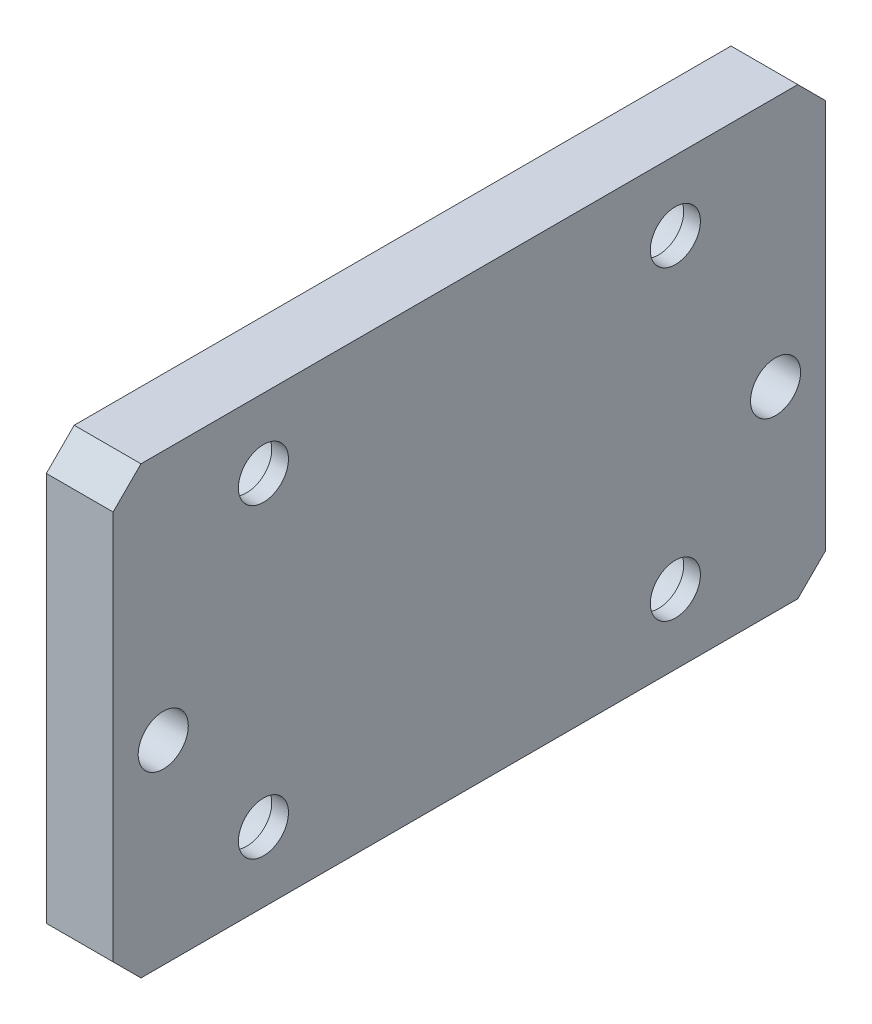
SolidWorks part; units mm, degrees
ref_plane "前视基准面" through (0, 0, 0) normal (0, 0, 1) x (1, 0, 0)
ref_plane "上视基准面" through (0, 0, 0) normal (0, 1, 0) x (1, 0, 0)
ref_plane "右视基准面" through (0, 0, 0) normal (1, 0, 0) x (0, 0, -1)
sketch "草图1" plane through (0, 0, 0) normal (1, 0, 0) x (0, 0, -1)
  line L1 (-64, 40) -> (64, 40)
  line L2 (-64, 40) -> (-64, -40)
  line L3 (-64, -40) -> (64, -40)
  line L4 (64, 40) -> (64, -40)
  line L5 (-64, 40) -> (64, -40) construction
  line L6 (-64, -40) -> (64, 40) construction
  point P0 (0, 0)
  dimension "D1" = 128
  dimension "D2" = 80
extrude "凸台-拉伸1" add sketch "草图1" along normal blind 12
hole_wizard "打孔尺寸(%根据)内六角圆柱头螺钉的类型1" positions "草图2" profile "草图3" counterbore size "M8" standard "GB" end condition through all
sketch "草图2" plane through (0, 0, 0) normal (-1, 0, 0) x (0, 0, 1)
  line L0 (0, 68.7616) -> (0, 0) construction
  line L1 (0, 0) -> (107.0716, 0) construction
  point P0 (-37, 27.5)
  point P2 (-37, -27.5)
  point P4 (37, 27.5)
  point P6 (37, -27.5)
  dimension "D1" = 55
  dimension "D2" = 74
sketch "草图3" plane through (0, 27.5, -37) normal (0, 1, 0) x (0, 0, 1)
  line L0 (0, 0) -> (0, 12)
  line L1 (0, 12) -> (4.5, 12)
  line L3 (4.5, 12) -> (4.5, 9)
  line L4 (4.5, 9) -> (7.5, 9)
  line L5 (7.5, 9) -> (7.5, 0)
  line L7 (7.5, 0) -> (0, 0)
  line L11 (0, -6.35) -> (0, 107.95) construction
  dimension "通孔孔直径" = 9
  dimension "通孔孔深度" = 12
  dimension "柱形沉头孔直径" = 15
  dimension "柱形沉头孔深度" = 9
hole_wizard "Ø9.0 (9) 直径孔1" positions "草图4" profile "草图5" hole size "Ø9.0" standard "GB" end condition through all
sketch "草图4" plane through (12, 0, 0) normal (1, 0, 0) x (0, 0, -1)
  line L0 (0, 68.4392) -> (0, -5) construction
  line L1 (0, -5) -> (89.928, -5) construction
  line L3 (64, 40) -> (-64, 40) construction
  point P2 (-55, -5)
  point P6 (55, -5)
  dimension "D1" = 110
  dimension "D2" = 45
sketch "草图5" plane through (12, -5, 55) normal (0, 1, 0) x (0, 0, -1)
  line L0 (0, 0) -> (0, 12)
  line L1 (0, 12) -> (4.5, 12)
  line L2 (4.5, 12) -> (4.5, 0)
  line L5 (4.5, 0) -> (0, 0)
  line L11 (0, -6.35) -> (0, 107.95) construction
  dimension "通孔孔直径" = 9
  dimension "通孔孔深度" = 12
chamfer "倒角1" distance 5 angle 45 4 edges at (6, -40, 64) (6, -40, -64) (6, 40, -64) (6, 40, 64)
